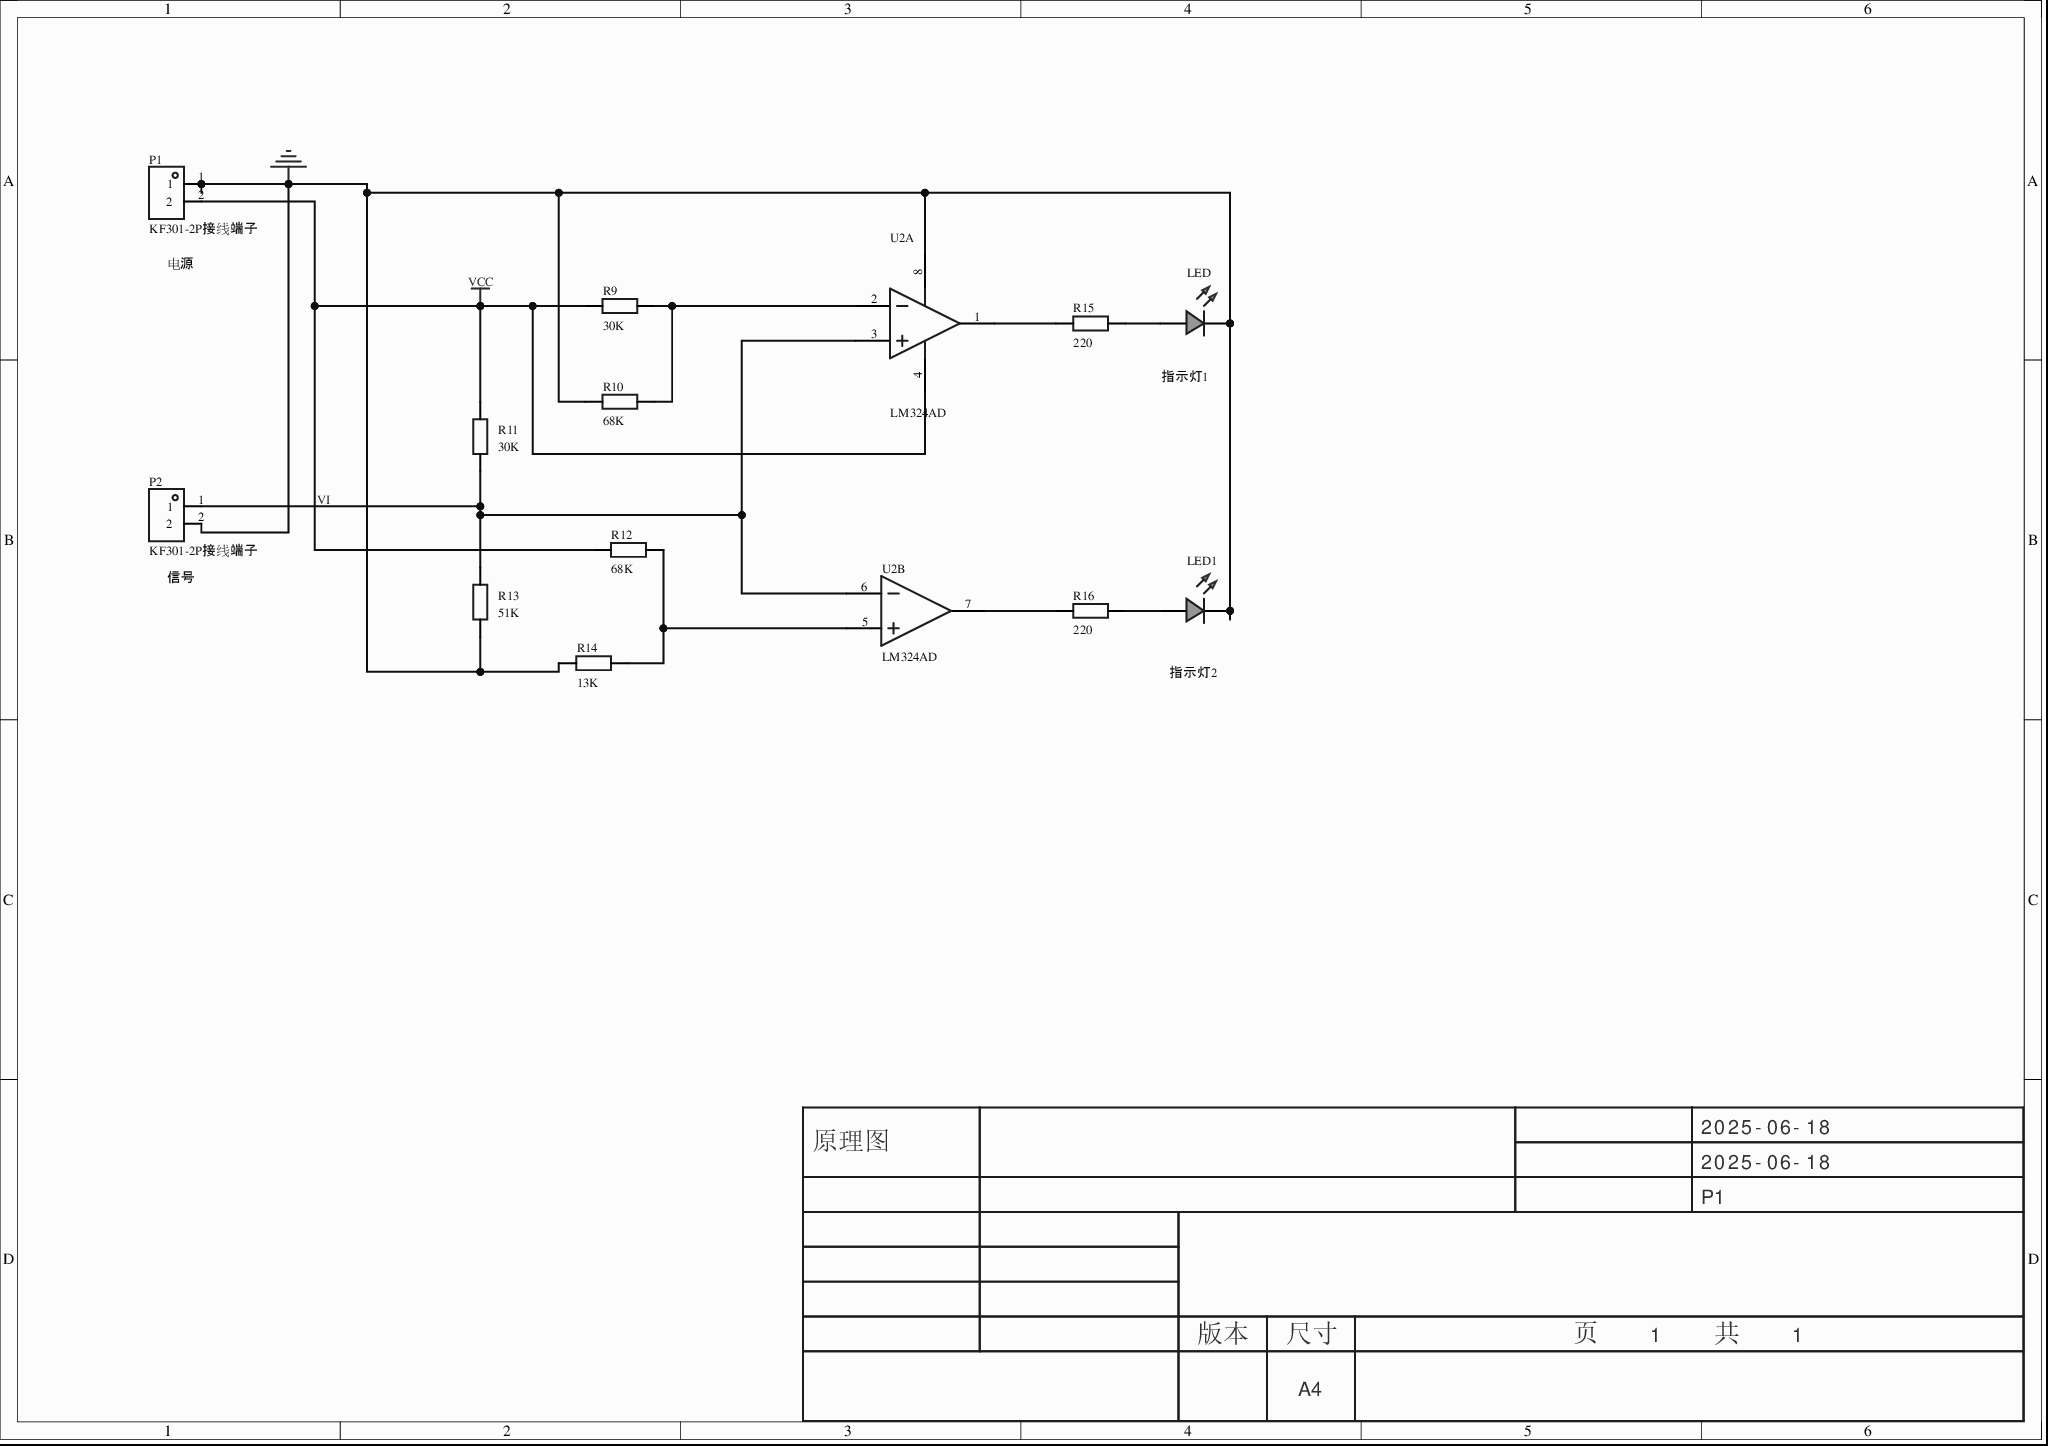
[diagram p0: MISC50866-3.schdoc]
# Altium project MISC50866-2.PrjPcb
1 sheet, 13 parts. Net scope: global (net labels, ports and power ports of the same name join across sheets).
Board file: MISC50866.pcbdoc

## Sheet MISC50866-3.schdoc
size 297 x 209 mm; Version: V1.0; @Project Name: MISC50866; @Page Count: 1; @Update Date: 2025-06-18; @Create Date: 2025-06-18; @Schematic Name: MISC50866; @Page No: 1; @Create Time: 22:17:12; @Update Time: 22:17:16; @Board Name: MISC50866

### Parts
LED  (no value)  [LED-TH_5mm]
LED1  (no value)  [LED-TH_5mm]
P1  KF301-2P接线端子  [CONN-TH_XY301V-A-5.0-2P]
P2  KF301-2P接线端子  [CONN-TH_XY301V-A-5.0-2P]
R9  30K  [Res_1/8W]
R10  68K  [Res_1/8W]
R11  30K  [Res_1/8W]
R12  68K  [Res_1/8W]
R13  51K  [Res_1/8W]
R14  13K  [Res_1/8W]
R15  220  [Res_1/8W]
R16  220  [Res_1/8W]
U2  LM324AD  [DIP-8_L9.3-W6.4-P2.54-LS7.6-BL]  (parts A,B of 2)

### Nets
GND: LED.2(A) LED1.2(A) P1.1 P2.2 R10.1 R13.1 R14.1 U2.8(VCC+)
VCC: P1.2 R9.1 R11.2 R12.1 U2.4(VCC-)
VI: P2.1 R11.1 R13.2 U2.3(IN1+) U2.6(IN2-)
NetLED1_1: LED1.1(C) R16.2
NetLED_1: LED.1(C) R15.2
NetR9_2: R9.2 R10.2 U2.2(IN1-)
NetR12_2: R12.2 R14.2 U2.5(IN2+)
NetR15_1: R15.1 U2.1(OUT1)
NetR16_1: R16.1 U2.7(OUT2)

### Notes on the sheet
- (near P1) 电源
- 指示灯1
- (near P2) 信号
- 指示灯2
- 2025-06-18
- 原理图
- P1
- 版本
- 尺寸
- A4
- 页    1    共    1

### Library data of the parts
LED LED1 = LED_TH-G_5mm: ConvertToPcb: yes; ModelId: fe7796f666a04da4b4289311169b45200819f05c4eef4c71ace90d822a990e87; ModelName: LED-TH_BD5.8-P2.54-FD_GREEN-1; ModelTransform: 212.58,227.91,537.36,0,0,0,-7.87,0,-196.85; Device: LED_TH-G_5mm; AddInBom: yes; Supplier Footprint: 插件; SymbolName: LED_TH-G; FootprintName: LED-TH_5mm
P1 P2 = KF301-2P接线端子: AddInBom: yes; ModelId: ef7ead88b0f2448d904975b26718870f; ModelTransform: 417.322,299.212,0,0,0,0,11.811,-7.835,-157.48; Symbol: KF301-2P接线端子; Device: KF301-2P接线端子; LCSC Part Name: KF301-2P接线端子; SupplierPart: C9900016950; ManufacturerPart: KF301-2P接线端子; Supplier Footprint: CK301-2P; Supplier: LCSC; ConvertToPcb: yes; FootprintName: CONN-TH_XY301V-A-5.0-2P; ModelName: CONN-TH_XY301V-A-5.0-2P
R9-R16 = Res_AXIAL-1/8W: ConvertToPcb: yes; SymbolName: 电阻; ModelId: b2b5ae7ae4c642178fe0039925c86a3f; ModelName: RES-TH_BD1.8-L3.2-P7.20-D0.4; ModelTransform: 282.86,66.88,253.09,0,0,0,0,0,-191; Device: Res_AXIAL-1/8W; AddInBom: yes; Supplier Footprint: 轴向引线; FootprintName: Res_1/8W
  R9 R11: Value: 30K
  R10 R12: Value: 68K
  R13: Value: 51K
  R14: Value: 13K
  R15 R16: Value: 220
U2 = NE5532N: 放大器数:双路;轨到轨:-;增益带宽积(GBP):10MHz;输入失调电压(Vos):5mV;压摆率(SR):11V/us;输入偏置电流(Ib):500nA;; Manufacturer: HGSEMI(华冠); Relevance: []; AddInBom: yes; ModelId: e1ba2ac1384341a197ae27979c8d8942; ModelName: DIP-8_L9.3-W6.4-H4.5-P2.54-LS7.6-BL; ModelTransform: 364.173,311.8104,0,0,0,0,0,0,-118.11; Number of Channels: 双路; Maximum Power Supply Range (Vdd-Vss): 44V; Gain Bandwidth Product: 10MHz; Vos - Input Offset Voltage: 5mV; Slew Rate: 11V/us; Ib - Input Bias Current: 500nA; Input Offset Current(Ios): 200nA; Noise density(eN): 8nV/√Hz@1kHz; Common Mode Rejection Ratio(CMRR): 100dB; Dual Supply: ±22V; Symbol: NE5532N; Manufacturer Part: LM324AD; Device: NE5532N; LCSC Part Name: NE5532N; SupplierPart: C2987282; Supplier Footprint: DIP-8; JLCPCB Part Class: 扩展库; Datasheet: https://atta.szlcsc.com/upload/public/pdf/source/20220420/2D3D2D023E04B50C3DA859F976397601.pdf; Supplier: LCSC; ConvertToPcb: yes; FootprintName: DIP-8_L9.3-W6.4-P2.54-LS7.6-BL; Rail to Rail: -; Input Offset Voltage Drift(Vos TC): -; Input offset current drift(Ios TC): -; Quiescent Current: -; Output Current: -; Operating Temperature: 0℃~+70℃; Single supply: -